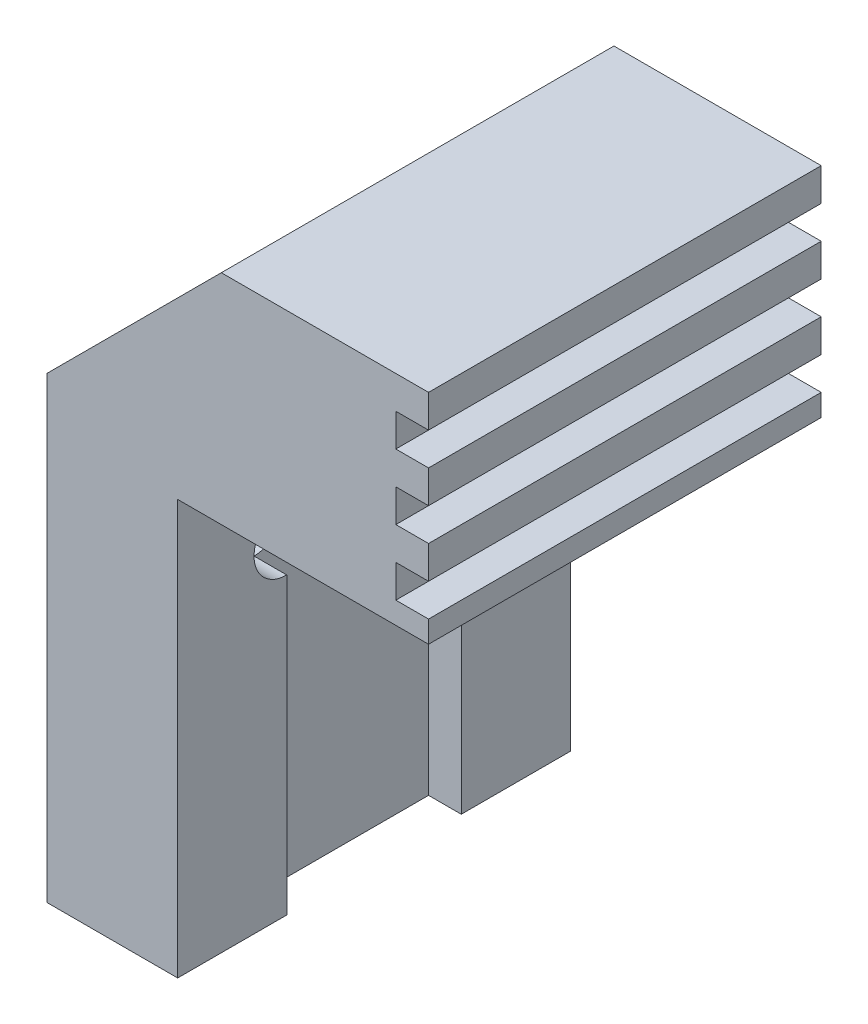
SolidWorks part; units mm, degrees
ref_plane "前视基准面" through (0, 0, 0) normal (0, 0, 1) x (1, 0, 0)
ref_plane "上视基准面" through (0, 0, 0) normal (0, 1, 0) x (1, 0, 0)
ref_plane "右视基准面" through (0, 0, 0) normal (1, 0, 0) x (0, 0, -1)
sketch "草图1" plane through (0, 0, 0) normal (0, 0, 1) x (1, 0, 0)
  line L0 (0, 0) -> (0, 29)
  line L1 (0, 29) -> (17.5, 29)
  line L2 (17.5, 29) -> (17.5, 19)
  line L3 (17.5, 19) -> (6, 19)
  line L4 (6, 19) -> (6, 0)
  line L5 (6, 0) -> (0, 0)
  dimension "D1" = 19
  dimension "D2" = 6
  dimension "D3" = 11.5
  dimension "D4" = 10
extrude "凸台-拉伸1" add sketch "草图1" along normal mid plane 18
sketch "草图2" plane through (6, 0, 0) normal (1, 0, 0) x (0, 0, -1)
  line L0 (-9, 0) -> (9, 0) construction
  line L1 (-4, 15) -> (4, 15)
  line L2 (-4, 15) -> (-4, 0)
  line L3 (-4, 0) -> (4, 0)
  line L4 (4, 15) -> (4, 0)
  line L5 (-4, 15) -> (4, 0) construction
  line L6 (-4, 0) -> (4, 15) construction
  point P0 (0, 7.5)
  dimension "D1" = 8
  dimension "D2" = 15
extrude "切除-拉伸1" cut sketch "草图2" against normal blind 1.5
sketch "草图3" plane through (6, 0, 0) normal (1, 0, 0) x (0, 0, -1)
  circle A0 centre (4, 15) radius 1.5
  circle A1 centre (-4, 15) radius 1.5
  dimension "D1" = 3
extrude "切除-拉伸2" cut sketch "草图3" against normal up to next
sketch "草图4" plane through (17.5, 0, 0) normal (1, 0, 0) x (0, 0, -1)
  line L0 (-9, 19) -> (-9, 29) construction
  line L1 (-9, 27.5) -> (9, 27.5)
  line L2 (-9, 27.5) -> (-9, 26)
  line L3 (-9, 26) -> (9, 26)
  line L4 (9, 27.5) -> (9, 26)
  line L5 (9, 19) -> (9, 29) construction
  line L6 (-9, 29) -> (9, 29) construction
  line L8 (-9, 23) -> (9, 23)
  line L9 (-9, 23) -> (-9, 24.5)
  line L10 (-9, 24.5) -> (9, 24.5)
  line L11 (9, 23) -> (9, 24.5)
  line L12 (-9, 20) -> (9, 20)
  line L13 (-9, 20) -> (-9, 21.5)
  line L14 (-9, 21.5) -> (9, 21.5)
  line L15 (9, 20) -> (9, 21.5)
extrude "切除-拉伸3" cut sketch "草图4" against normal blind 1.5
chamfer "倒角1" distance 8 angle 45 1 edges at (0, 29, 0)
equation "\"D4@草图4\"=\"D3@草图4\""
